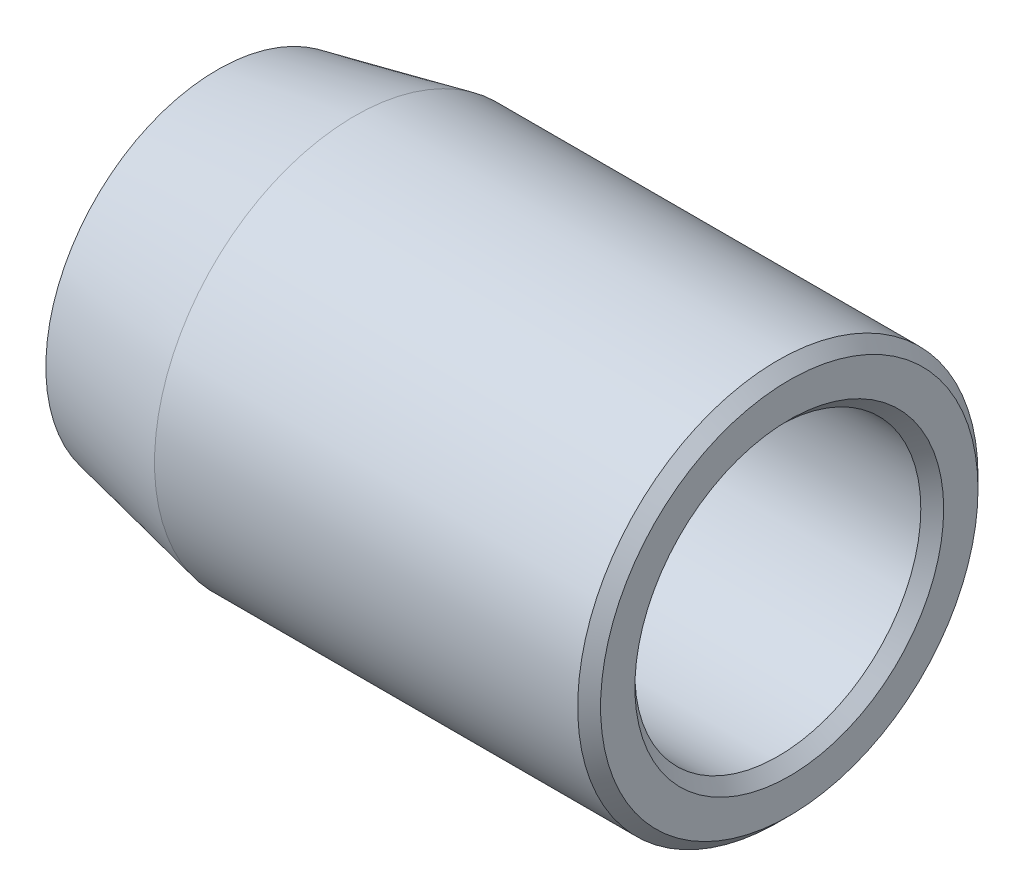
SolidWorks part; units mm, degrees
material "Q235A"
ref_plane "Front Plane" through (0, 0, 0) normal (0, 0, 1) x (1, 0, 0)
ref_plane "Top Plane" through (0, 0, 0) normal (0, 1, 0) x (1, 0, 0)
ref_plane "Right Plane" through (0, 0, 0) normal (1, 0, 0) x (0, 0, -1)
sketch "Sketch1" plane through (0, 0, 0) normal (0, 0, 1) x (1, 0, 0)
  line L0 (0, 0) -> (-72.7314, 0) construction
  line L1 (0, 12.5) -> (0, 17.5)
  line L2 (0, 17.5) -> (-38, 17.5)
  line L3 (-38, 17.5) -> (-50, 15)
  line L4 (-50, 15) -> (-50, 12.5)
  line L5 (-50, 12.5) -> (0, 12.5)
  point P9 (0, 15)
  dimension "D1" = 25
  dimension "D2" = 35
  dimension "D3" = 30
  dimension "D4" = 50
  dimension "D5" = 38
revolve "Revolve1" add sketch "Sketch1" angle 360 about L0
chamfer "Chamfer1" distance 1 angle 45 2 edges at (0, 0, -17.5) (0, 0, -12.5)
